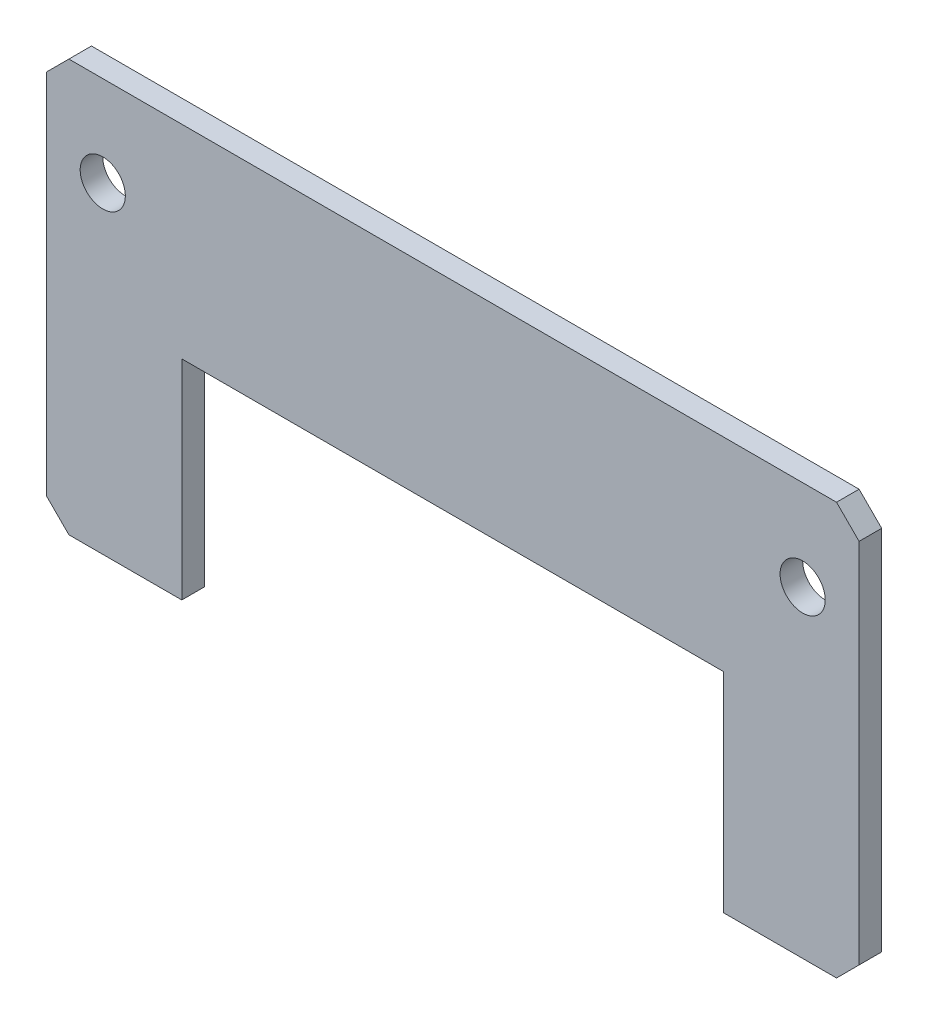
from build123d import *

# Parameters (mm, degrees)
SKETCH1_W               = 720
SKETCH1_H               = 365
BOSS_EXTRUDE1_DEPTH     = 20
CUT_EXTRUDE1_DEPTH      = 405.111680108
CUT_EXTRUDE1_DEPTH_BACK = 405.111680108
SKETCH2_R               = 20
CHAMFER1_SIZE           = 20
CHAMFER2_SIZE           = 20
CUT_EXTRUDE2_DEPTH      = 405.111680108
CUT_EXTRUDE2_DEPTH_BACK = 405.111680108
SKETCH4_W               = 480
SKETCH4_H               = 370


with BuildPart() as part:
    # Sketch1 → Boss-Extrude1 (new body)
    with BuildSketch(Plane.XY):
        Rectangle(SKETCH1_W, SKETCH1_H)
    extrude(amount=BOSS_EXTRUDE1_DEPTH)

    # Sketch2 → Cut-Extrude1 (cut, two sides: drawn at the far end of the back side and taken through both)
    with BuildSketch(Plane.XY.offset(20).offset(-CUT_EXTRUDE1_DEPTH_BACK)):
        with Locations((-310, 102.5)):
            Circle(SKETCH2_R)
        with Locations((310, 102.5)):
            Circle(SKETCH2_R)
    extrude(amount=CUT_EXTRUDE1_DEPTH + CUT_EXTRUDE1_DEPTH_BACK, mode=Mode.SUBTRACT)

    # Chamfer1
    chamfer1_edges = [part.edges().sort_by_distance(p)[0] for p in [
        (-360, 182.5, 10),
        (360, 182.5, 10),
    ]]
    chamfer(chamfer1_edges, length=CHAMFER1_SIZE)

    # Chamfer2
    chamfer2_edges = [part.edges().sort_by_distance(p)[0] for p in [
        (360, -182.5, 10),
        (-360, -182.5, 10),
    ]]
    chamfer(chamfer2_edges, length=CHAMFER2_SIZE)

    # Sketch4 → Cut-Extrude2 (cut, two sides: drawn at the far end of the back side and taken through both)
    with BuildSketch(Plane.XY.offset(20).offset(-CUT_EXTRUDE2_DEPTH_BACK)):
        with Locations((0, -182.5)):
            Rectangle(SKETCH4_W, SKETCH4_H)
    extrude(amount=CUT_EXTRUDE2_DEPTH + CUT_EXTRUDE2_DEPTH_BACK, mode=Mode.SUBTRACT)


solid = part.part
